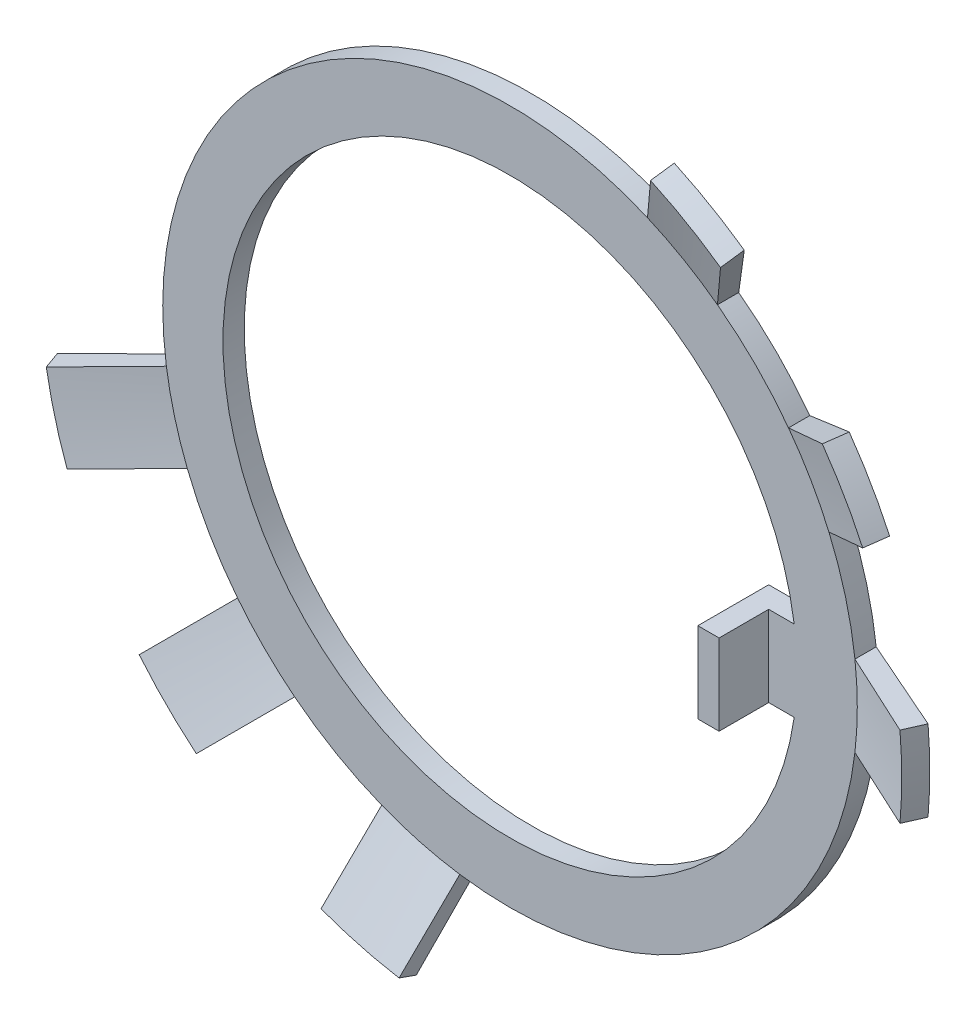
from build123d import *

# Parameters (mm, degrees)
SKETCH2_OUTSIDE_W = 81.556
SKETCH2_OUTSIDE_H = 81.556
CUT_EXTRUDE_DEPTH = 47.45561719
SKETCH4_W         = 5.7
SKETCH4_H         = 3.5
EXTRUDE1_DEPTH    = 1.5


with BuildPart() as part:
    # Sketch1 → Base-Extrude (revolve)
    with BuildSketch(Plane.YZ, mode=Mode.PRIVATE) as base_extrude_sk:
        Polygon((0, -4.247960103), (-24.5, -4.247960103), (-31, -1.371705006), (-30.393019459, 0), (-24.5, -2.747960103), (0, -2.747960103), align=None)
    revolve(base_extrude_sk.sketch.rotate(Axis((0, 0, 5.823648763), (0, 0, -1)), 270), axis=Axis((0, 0, 5.823648763), (0, 0, -1)))

    # Sketch2 outside → Cut-Extrude (cut, through all)
    # profile 1 of 2: a face of its own
    with BuildSketch(Plane(origin=(-2.40435344, 1.003568156, -4.247960103), x_dir=(-1, 0, 0), z_dir=(0, 0, -1))):
        with Locations((-2.404, -1.004)):
            Rectangle(SKETCH2_OUTSIDE_W, SKETCH2_OUTSIDE_H)
        with BuildLine():
            Line((-26.738023529, -3.853568156), (-33.273067375, -3.853568156))
            ThreePointArc((-33.273067375, -3.853568156), (-33.40435344, -1.003568156), (-33.273067375, 1.846431844))
            Line((-33.273067375, 1.846431844), (-26.738023529, 1.846431844))
            ThreePointArc((-26.738023529, 1.846431844), (-26.069536184, 5.337498449), (-24.902929904, 8.695094487))
            Line((-24.902929904, 8.695094487), (-30.562443889, 11.96261641))
            ThreePointArc((-30.562443889, 11.96261641), (-29.251140957, 14.496431844), (-27.712443889, 16.898961212))
            Line((-27.712443889, 16.898961212), (-22.052929904, 13.631439289))
            ThreePointArc((-22.052929904, 13.631439289), (-19.728469579, 16.320547983), (-17.039360885, 18.645008308))
            Line((-17.039360885, 18.645008308), (-20.306882808, 24.304522293))
            ThreePointArc((-20.306882808, 24.304522293), (-17.90435344, 25.843219361), (-15.370538006, 27.154522293))
            Line((-15.370538006, 27.154522293), (-12.103016083, 21.495008308))
            ThreePointArc((-12.103016083, 21.495008308), (12.510301571, 18.433588681), (21.837801226, -4.548696808))
            Line((21.837801226, -4.548696808), (28.150168853, -6.240090616))
            ThreePointArc((28.150168853, -6.240090616), (27.539347175, -9.026958555), (26.674900296, -11.745867825))
            Line((26.674900296, -11.745867825), (20.362532669, -10.054474018))
            ThreePointArc((20.362532669, -10.054474018), (18.813268953, -13.253568156), (16.817404018, -16.194816961))
            Line((16.817404018, -16.194816961), (21.438377837, -20.81579078))
            ThreePointArc((21.438377837, -20.81579078), (19.515956777, -22.923878373), (17.407869184, -24.846299433))
            Line((17.407869184, -24.846299433), (12.786895365, -20.225325614))
            ThreePointArc((12.786895365, -20.225325614), (9.84564656, -22.221190549), (6.646552422, -23.770454265))
            Line((6.646552422, -23.770454265), (8.33794623, -30.082821892))
            ThreePointArc((8.33794623, -30.082821892), (5.619036959, -30.947268771), (2.83216902, -31.558090449))
            Line((2.83216902, -31.558090449), (1.140775212, -25.245722822))
            ThreePointArc((1.140775212, -25.245722822), (-17.31900845, -20.440724994), (-26.738023529, -3.853568156))
        make_face(mode=Mode.SUBTRACT)
    # profile 2 of 2: a face of its own
    with BuildSketch(Plane(origin=(-2.40435344, 1.003568156, -4.247960103), x_dir=(-1, 0, 0), z_dir=(0, 0, -1))):
        with BuildLine():
            Line((-22.452794776, 1.846431844), (-19.15435344, 1.846431844))
            Line((-19.15435344, 1.846431844), (-19.15435344, -3.853568156))
            Line((-19.15435344, -3.853568156), (-22.452794776, -3.853568156))
            ThreePointArc((-22.452794776, -3.853568156), (17.84564656, -1.003568156), (-22.452794776, 1.846431844))
        make_face()
    extrude(amount=-CUT_EXTRUDE_DEPTH, mode=Mode.SUBTRACT)

    # Sketch4 → Extrude1 (add)
    with BuildSketch(Plane(origin=(16.75, -0.667304961, -0.255028377), x_dir=(0, 1, 0), z_dir=(-1, 0, 0))):
        with Locations((0.667304961, 0.742931726)):
            Rectangle(SKETCH4_W, SKETCH4_H)
    extrude(amount=-EXTRUDE1_DEPTH)


solid = part.part
